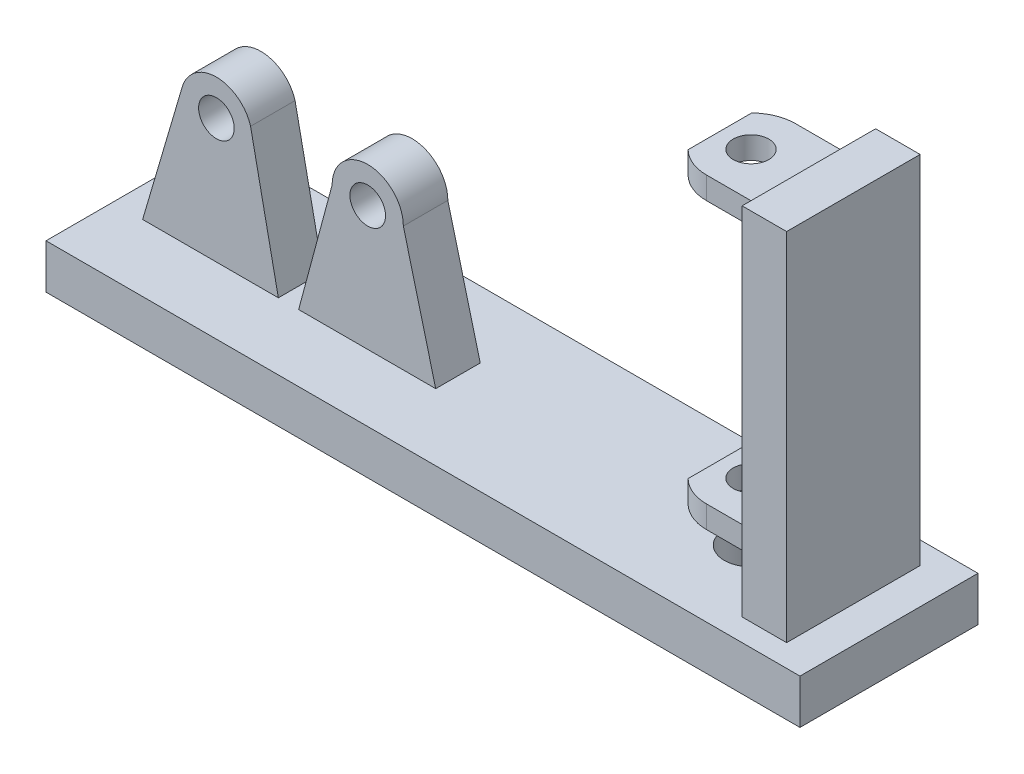
from build123d import *

# Parameters (mm, degrees)
SKETCH1_R           = 4
BOSS_EXTRUDE1_DEPTH = 10
SKETCH2_W           = 169.403995176
SKETCH2_H           = 40
BOSS_EXTRUDE2_DEPTH = 10
SKETCH3_W           = 10
SKETCH3_H           = 30
BOSS_EXTRUDE3_DEPTH = 80
SKETCH4_W           = 20
SKETCH4_H           = 5
BOSS_EXTRUDE4_DEPTH = 20
SKETCH5_R           = 4
CUT_EXTRUDE1_DEPTH  = 70
SKETCH6_R           = 6
CUT_EXTRUDE2_DEPTH  = 30


with BuildPart() as part:
    # Sketch1 → Boss-Extrude1 (new body)
    with BuildSketch(Plane.XY):
        with BuildLine():
            Line((-7.674547775, 2.258609406), (-16.579617078, -28))
            Line((-16.579617078, -28), (-22.35311977, -38))
            Line((-22.35311977, -38), (137.64688023, -38))
            Line((137.64688023, -38), (131.873377539, -28))
            Line((131.873377539, -28), (49.354955752, -28.3172709))
            Line((49.354955752, -28.3172709), (42, 0))
            ThreePointArc((42, 0), (34, 8), (26, 0))
            Line((26, 0), (18.4767103, -28))
            Line((18.4767103, -28), (13.916688293, -28))
            Line((13.916688293, -28), (7.674547775, 2.258609406))
            ThreePointArc((7.674547775, 2.258609406), (0, 8), (-7.674547775, 2.258609406))
        make_face()
        Circle(SKETCH1_R, mode=Mode.SUBTRACT)
        with Locations((34, 0)):
            Circle(SKETCH1_R, mode=Mode.SUBTRACT)
    extrude(amount=BOSS_EXTRUDE1_DEPTH)

    # Sketch2 → Boss-Extrude2 (add)
    with BuildSketch(Plane(origin=(0, -38, 0), x_dir=(-1, 0, 0), z_dir=(0, -1, 0))):
        with Locations((-61.414188083, -5)):
            Rectangle(SKETCH2_W, SKETCH2_H)
    extrude(amount=-BOSS_EXTRUDE2_DEPTH)

    # Sketch3 → Boss-Extrude3 (add)
    with BuildSketch(Plane(origin=(0, -28, 0), x_dir=(1, 0, 0), z_dir=(0, 1, 0))):
        with Locations((133.116185671, -5)):
            Rectangle(SKETCH3_W, SKETCH3_H)
    extrude(amount=BOSS_EXTRUDE3_DEPTH)

    # Sketch4 → Boss-Extrude4 (add)
    with BuildSketch(Plane.ZY.offset(-128.116185671)):
        with Locations((5, 46.5)):
            Rectangle(SKETCH4_W, SKETCH4_H)
        with Locations((5, -17.5)):
            Rectangle(SKETCH4_W, SKETCH4_H)
    extrude(amount=BOSS_EXTRUDE4_DEPTH)

    # Sketch5 → Cut-Extrude1 (cut)
    with BuildSketch(Plane(origin=(0, 49, 0), x_dir=(1, 0, 0), z_dir=(0, 1, 0))):
        with Locations(Location((115.116185671, -5, 0), (0, 0, 270))):
            Circle(SKETCH5_R)
        with BuildLine():
            Line((115.116185671, -15), (103.174329038, -18.113908317))
            Line((103.174329038, -18.113908317), (97.147243506, 5))
            Line((97.147243506, 5), (115.116185671, 5))
            ThreePointArc((115.116185671, 5), (105.116185671, -5), (115.116185671, -15))
        make_face()
    extrude(amount=-CUT_EXTRUDE1_DEPTH, mode=Mode.SUBTRACT)

    # Sketch6 → Cut-Extrude2 (cut)
    with BuildSketch(Plane(origin=(0, -28, 0), x_dir=(1, 0, 0), z_dir=(0, 1, 0))):
        with Locations(Location((115.116185671, -5, 0), (0, 0, 270))):
            Circle(SKETCH6_R)
    extrude(amount=-CUT_EXTRUDE2_DEPTH, mode=Mode.SUBTRACT)


solid = part.part
